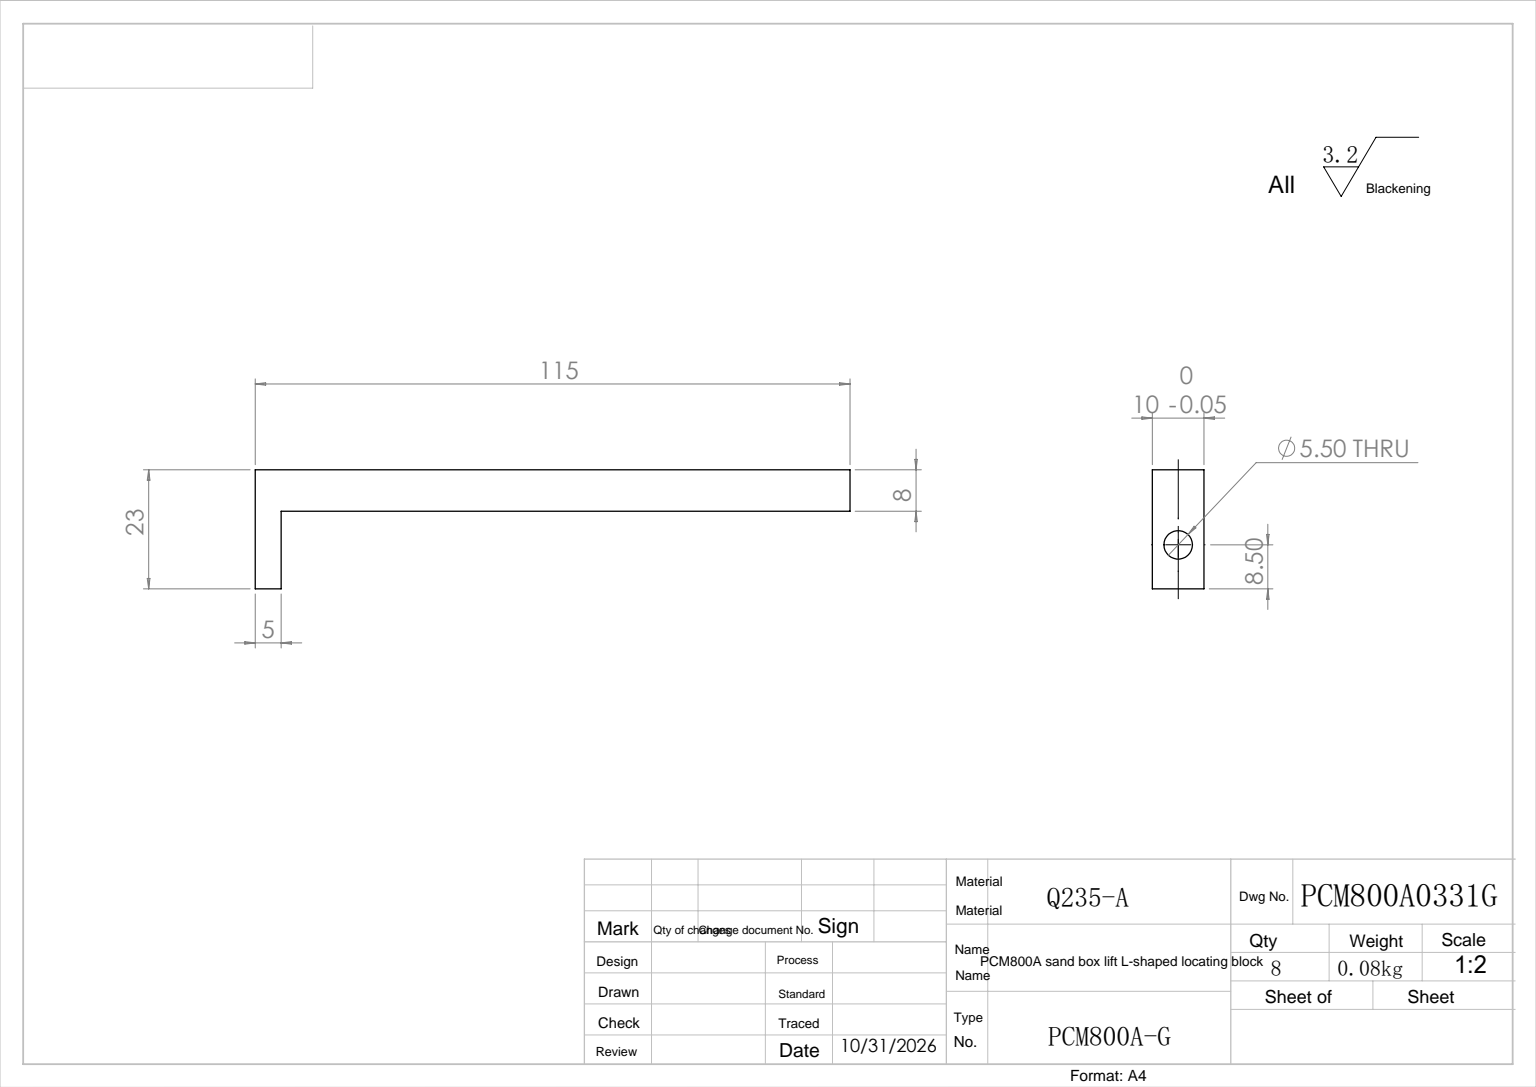
SolidWorks part; units mm, degrees
ref_plane "前视基准面" through (0, 0, 0) normal (0, 0, 1) x (1, 0, 0)
ref_plane "上视基准面" through (0, 0, 0) normal (0, 1, 0) x (1, 0, 0)
ref_plane "右视基准面" through (0, 0, 0) normal (1, 0, 0) x (0, 0, -1)
sketch "草图1" plane through (0, 0, 0) normal (0, 0, 1) x (1, 0, 0)
  line L0 (0, 0) -> (0, -110)
  line L1 (0, -110) -> (15, -110)
  line L2 (-8, 0) -> (-8, -115)
  line L3 (15, -110) -> (15, -115)
  line L4 (-8, 0) -> (0, 0)
  line L5 (0, 0) -> (0.1509, -0.1427)
  line L6 (15, -115) -> (-8, -115)
  line L7 (-8, -118) -> (15, -118) construction
  line L9 (-8, 0) -> (-8, -118) construction
  dimension "D1" = 110
  dimension "D2" = 23
  dimension "D3" = 8
  dimension "D4" = 5
extrude "凸台-拉伸1" add sketch "草图1" along normal blind 10
sketch "草图2" plane through (0, -115, 0) normal (0, -1, 0) x (1, 0, 0)
  line L2 (15, 10) -> (15, 0) construction
  line L3 (15, 10) -> (-8, 10) construction
  circle A0 centre (6.5, 5) radius 2.75
  dimension "D1" = 5.5
  dimension "D3" = 5
  dimension "D2" = 8.5
extrude "切除-拉伸1" cut sketch "草图2" against normal through all
